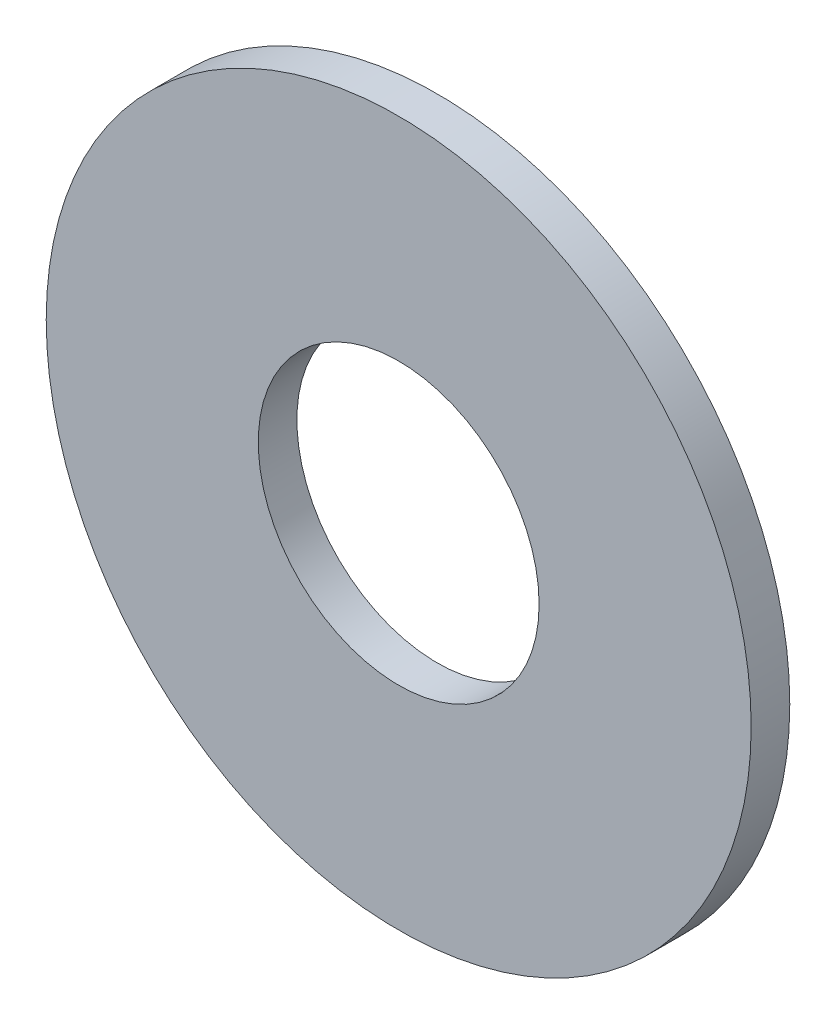
from build123d import *

# Parameters (mm, degrees)
SKETCH1_R           = 16.002
SKETCH1_R_2         = 6.3754
BOSS_EXTRUDE1_DEPTH = 1.7526


with BuildPart() as part:
    # Sketch1 → Boss-Extrude1 (new body)
    with BuildSketch(Plane.XY):
        Circle(SKETCH1_R)
        Circle(SKETCH1_R_2, mode=Mode.SUBTRACT)
    extrude(amount=BOSS_EXTRUDE1_DEPTH)


solid = part.part
